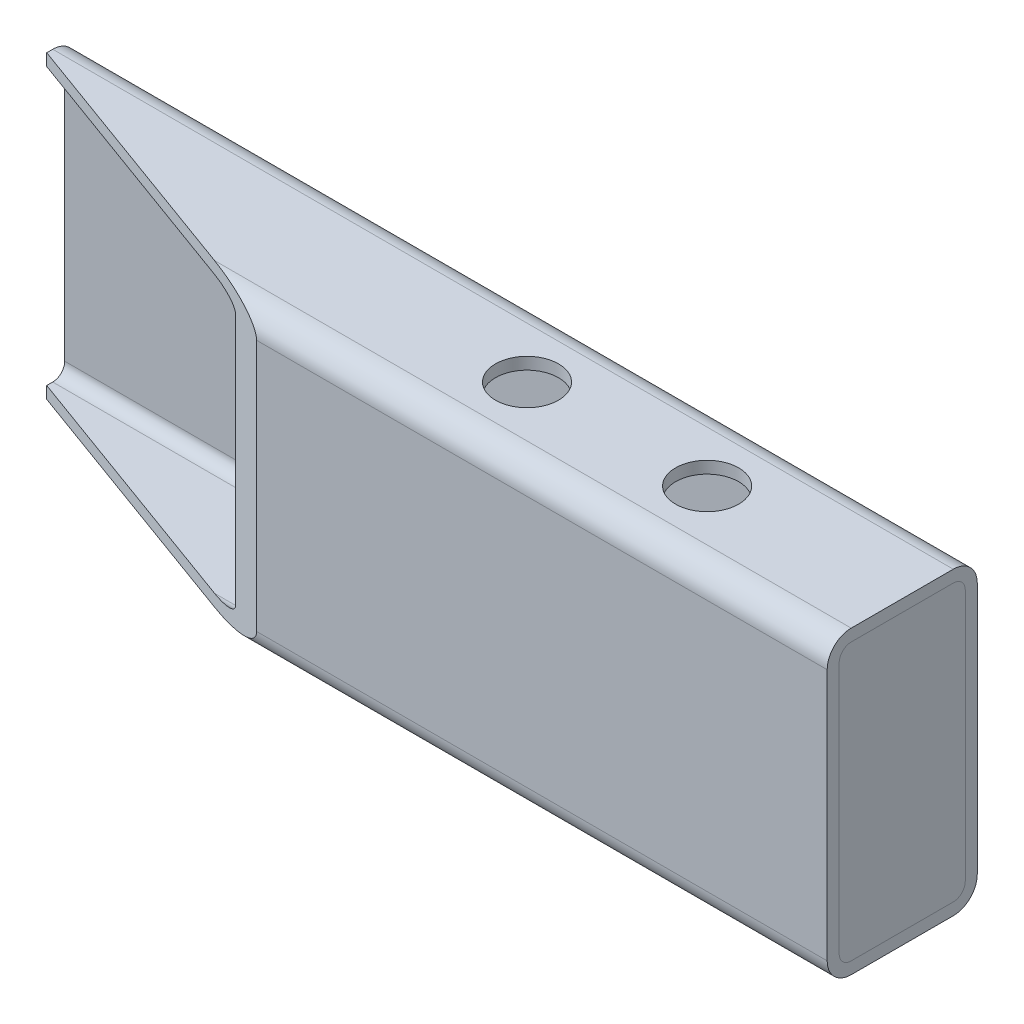
from build123d import *

# Parameters (mm, degrees)
F_100_X_50_X_4_1_DEPTH = 300
CUT_EXTRUDE_1_REACH    = 319.214
SKETCH_2_R             = 10.5
EXTRUDE_1_DEPTH        = 25


with BuildPart() as part:
    # Sketch1 → 矩形管 100 X 50 X 4(1) (new body)
    with BuildSketch(Plane(origin=(0, 0, 0), x_dir=(0, 0, -1), z_dir=(1, 0, 0))):
        with BuildLine():
            Line((-17, -50), (17, -50))
            ThreePointArc((17, -50), (22.656854249, -47.656854249), (25, -42))
            Line((25, -42), (25, 42))
            ThreePointArc((25, 42), (22.656854249, 47.656854249), (17, 50))
            Line((17, 50), (-17, 50))
            ThreePointArc((-17, 50), (-22.656854249, 47.656854249), (-25, 42))
            Line((-25, 42), (-25, -42))
            ThreePointArc((-25, -42), (-22.656854249, -47.656854249), (-17, -50))
        make_face()
        with BuildLine():
            Line((-17, -46), (17, -46))
            ThreePointArc((17, -46), (19.828427125, -44.828427125), (21, -42))
            Line((21, -42), (21, 42))
            ThreePointArc((21, 42), (19.828427125, 44.828427125), (17, 46))
            Line((17, 46), (-17, 46))
            ThreePointArc((-17, 46), (-19.828427125, 44.828427125), (-21, 42))
            Line((-21, 42), (-21, -42))
            ThreePointArc((-21, -42), (-19.828427125, -44.828427125), (-17, -46))
        make_face(mode=Mode.SUBTRACT)
    extrude(amount=F_100_X_50_X_4_1_DEPTH)

    # 切除-拉伸1: up to this face of the body (flat: up to its plane)
    cut_extrude_1_end = Plane(part.part.faces().sort_by_distance((150, 50, 0))[0])
    # 草图2 → 切除-拉伸1 (cut, up to the picked face)
    with BuildSketch(Plane.XZ.offset(50), mode=Mode.PRIVATE) as cut_extrude_1_sk1:
        with Locations(Location((235, 0, 0), (0, 0, 270))):
            Circle(SKETCH_2_R)
    cut_extrude_1_tool1 = split(extrude(cut_extrude_1_sk1.sketch, amount=-CUT_EXTRUDE_1_REACH, mode=Mode.PRIVATE), bisect_by=cut_extrude_1_end, keep=Keep.BOTH, mode=Mode.PRIVATE)
    # 草图2 → 切除-拉伸1 (cut, up to the picked face)
    with BuildSketch(Plane.XZ.offset(50), mode=Mode.PRIVATE) as cut_extrude_1_sk2:
        with Locations(Location((175, 0, 0), (0, 0, 270))):
            Circle(SKETCH_2_R)
    cut_extrude_1_tool2 = split(extrude(cut_extrude_1_sk2.sketch, amount=-CUT_EXTRUDE_1_REACH, mode=Mode.PRIVATE), bisect_by=cut_extrude_1_end, keep=Keep.BOTH, mode=Mode.PRIVATE)
    # 草图2 → 切除-拉伸1 (cut, up to the picked face)
    with BuildSketch(Plane.XZ.offset(50), mode=Mode.PRIVATE) as cut_extrude_1_sk3:
        Polygon((0, -15), (109.899096778, 25), (0, 25), align=None)
    cut_extrude_1_tool3 = split(extrude(cut_extrude_1_sk3.sketch, amount=-CUT_EXTRUDE_1_REACH, mode=Mode.PRIVATE), bisect_by=cut_extrude_1_end, keep=Keep.BOTH, mode=Mode.PRIVATE)
    add(cut_extrude_1_tool1.solids().sort_by(Axis((235, -50, 0), (0, 1, 0)))[0], mode=Mode.SUBTRACT)
    add(cut_extrude_1_tool2.solids().sort_by(Axis((175, -50, 0), (0, 1, 0)))[0], mode=Mode.SUBTRACT)
    add(cut_extrude_1_tool3.solids().sort_by(Axis((36.633032, -50, 11.666667), (0, 1, 0)))[0], mode=Mode.SUBTRACT)


with BuildPart() as body_2:
    # 草图3 → 凸台-拉伸1 (new body)
    with BuildSketch(Plane(origin=(300, 0, 0), x_dir=(0, 0, -1), z_dir=(1, 0, 0))):
        with BuildLine():
            Line((-17, 46), (17, 46))
            ThreePointArc((17, 46), (19.828427125, 44.828427125), (21, 42))
            Line((21, 42), (21, -42))
            ThreePointArc((21, -42), (19.828427125, -44.828427125), (17, -46))
            Line((17, -46), (-17, -46))
            ThreePointArc((-17, -46), (-19.828427125, -44.828427125), (-21, -42))
            Line((-21, -42), (-21, 42))
            ThreePointArc((-21, 42), (-19.828427125, 44.828427125), (-17, 46))
        make_face()
    extrude(amount=-EXTRUDE_1_DEPTH)


solid = Compound([part.part, body_2.part])
